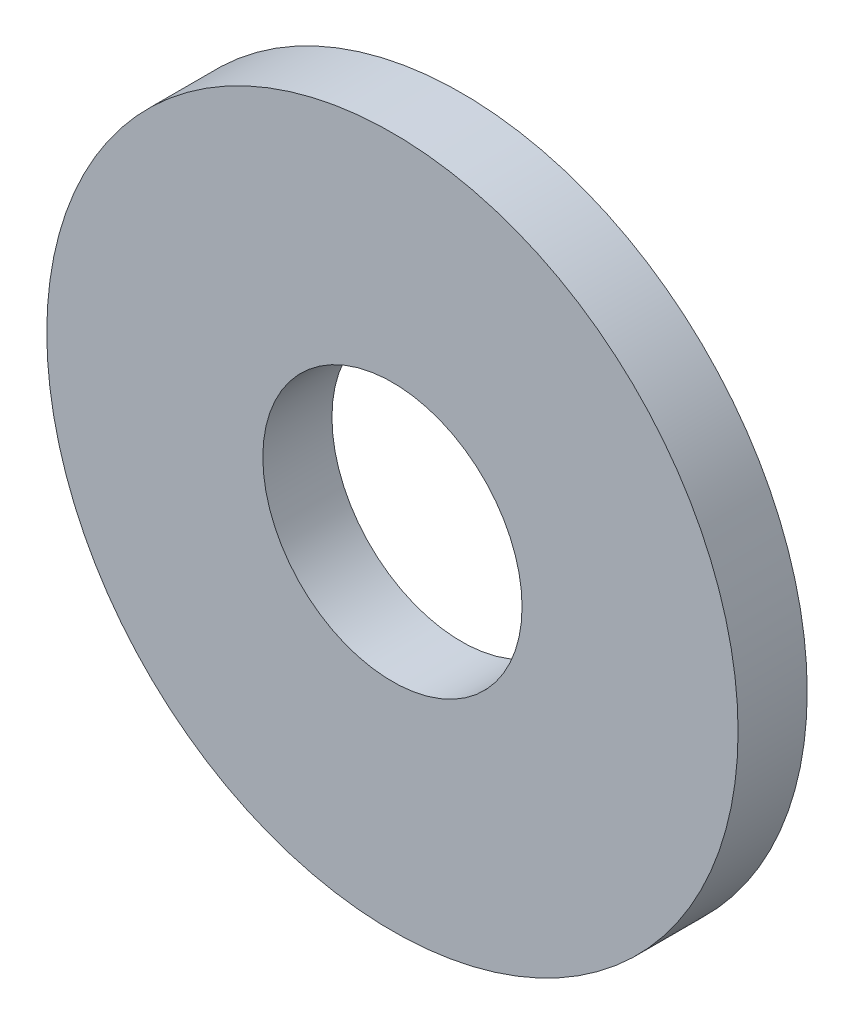
from build123d import *

# Parameters (mm, degrees)
SKETCH1_R           = 20
SKETCH1_R_2         = 7.5
BOSS_EXTRUDE1_DEPTH = 4


with BuildPart() as part:
    # Sketch1 → Boss-Extrude1 (new body)
    with BuildSketch(Plane.XY):
        Circle(SKETCH1_R)
        Circle(SKETCH1_R_2, mode=Mode.SUBTRACT)
    extrude(amount=BOSS_EXTRUDE1_DEPTH)


solid = part.part
